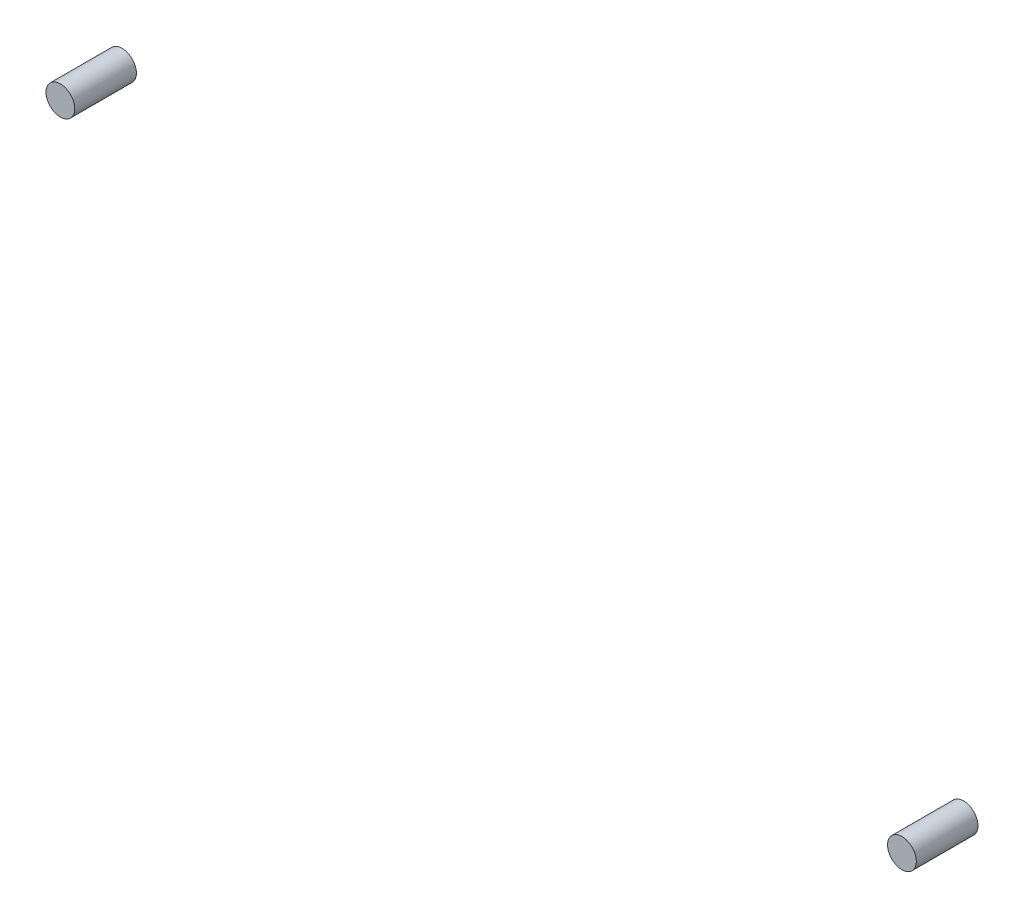
from build123d import *

# Parameters (mm, degrees)
SKETCH1_R             = 7
BOSS_EXTRUDE1_DEPTH   = 30
BOSS_EXTRUDE1_2_DEPTH = 30


with BuildPart() as part:
    # Sketch1 → Boss-Extrude1 (new body)
    with BuildSketch(Plane.XY):
        with Locations((629, 379.877558602)):
            Circle(SKETCH1_R)
    extrude(amount=BOSS_EXTRUDE1_DEPTH)


with BuildPart() as body_2:
    # Sketch1 → Boss-Extrude1 2 (new body)
    with BuildSketch(Plane.XY):
        with Locations((219.565172816, 492.277558602)):
            Circle(SKETCH1_R)
    extrude(amount=BOSS_EXTRUDE1_2_DEPTH)


solid = Compound([part.part, body_2.part])
